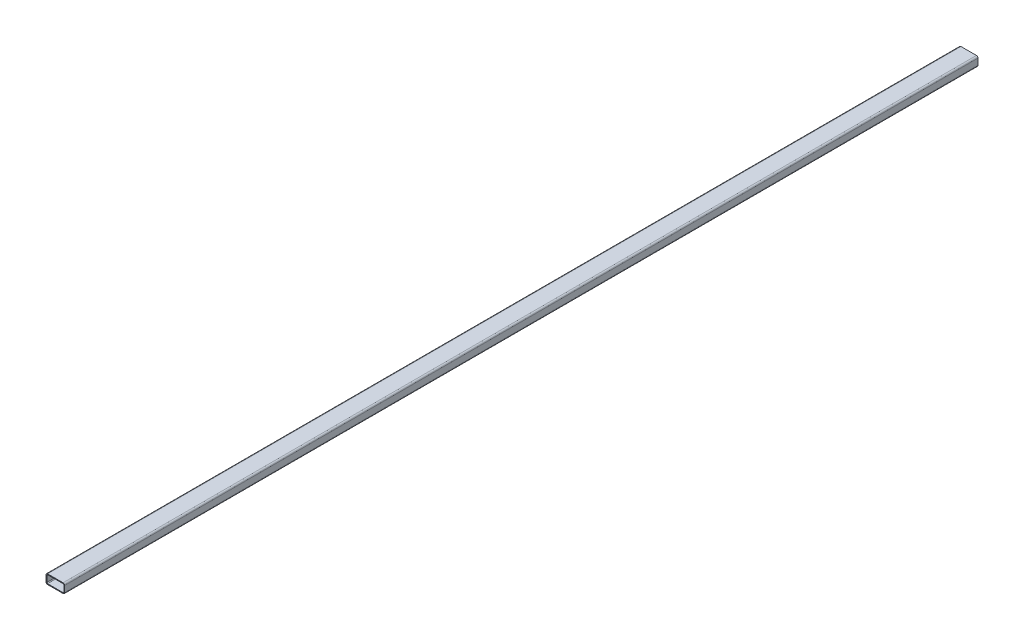
from build123d import *

# Parameters (mm, degrees)
BOSS_EXTRUDE1_DEPTH = 5880


with BuildPart() as part:
    # Sketch1 → Boss-Extrude1 (new body)
    with BuildSketch(Plane.XY):
        with BuildLine():
            Line((10, 0), (110, 0))
            ThreePointArc((110, 0), (117.071067812, 2.928932188), (120, 10))
            Line((120, 10), (120, 50))
            ThreePointArc((120, 50), (117.071067812, 57.071067812), (110, 60))
            Line((110, 60), (10, 60))
            ThreePointArc((10, 60), (2.928932188, 57.071067812), (0, 50))
            Line((0, 50), (0, 10))
            ThreePointArc((0, 10), (2.928932188, 2.928932188), (10, 0))
        make_face()
        with BuildLine():
            Line((10, 55), (110, 55))
            ThreePointArc((110, 55), (113.535533906, 53.535533906), (115, 50))
            Line((115, 50), (115, 10))
            ThreePointArc((115, 10), (113.535533906, 6.464466094), (110, 5))
            Line((110, 5), (10, 5))
            ThreePointArc((10, 5), (6.464466094, 6.464466094), (5, 10))
            Line((5, 10), (5, 50))
            ThreePointArc((5, 50), (6.464466094, 53.535533906), (10, 55))
        make_face(mode=Mode.SUBTRACT)
    extrude(amount=BOSS_EXTRUDE1_DEPTH)


solid = part.part
